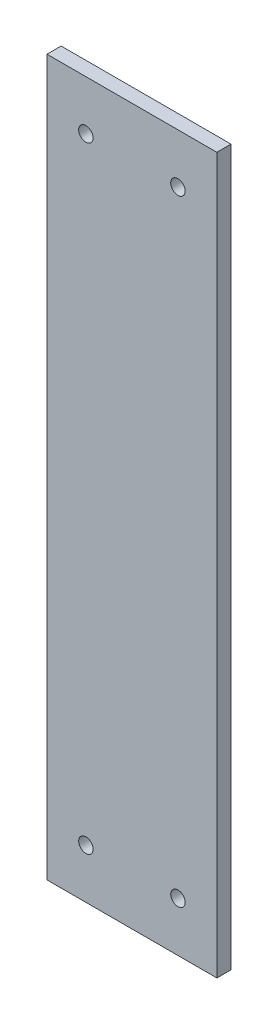
from build123d import *

# Parameters (mm, degrees)
SKETCH1_W              = 120
SKETCH1_H              = 505
BOSS_EXTRUDE1_DEPTH    = 10
M12_TAPPED_HOLE1_D     = 10.2
M12_TAPPED_HOLE1_DEPTH = 29.25
M12_TAPPED_HOLE1_TIP   = 3.064389157


with BuildPart() as part:
    # Sketch1 → Boss-Extrude1 (new body)
    with BuildSketch(Plane.XY):
        Rectangle(SKETCH1_W, SKETCH1_H)
    extrude(amount=BOSS_EXTRUDE1_DEPTH)

    # M12 Tapped Hole1
    with Locations(Plane.XY.offset(10)):
        with Locations((-32.5, 217.5), (32.5, 217.5), (32.5, -217.5), (-32.5, -217.5)):
            Hole(M12_TAPPED_HOLE1_D / 2, depth=M12_TAPPED_HOLE1_DEPTH)
            with Locations((0, 0, -(M12_TAPPED_HOLE1_DEPTH + M12_TAPPED_HOLE1_TIP / 2))):  # 118° drill point
                Cone(0, M12_TAPPED_HOLE1_D / 2, M12_TAPPED_HOLE1_TIP, mode=Mode.SUBTRACT)


solid = part.part
